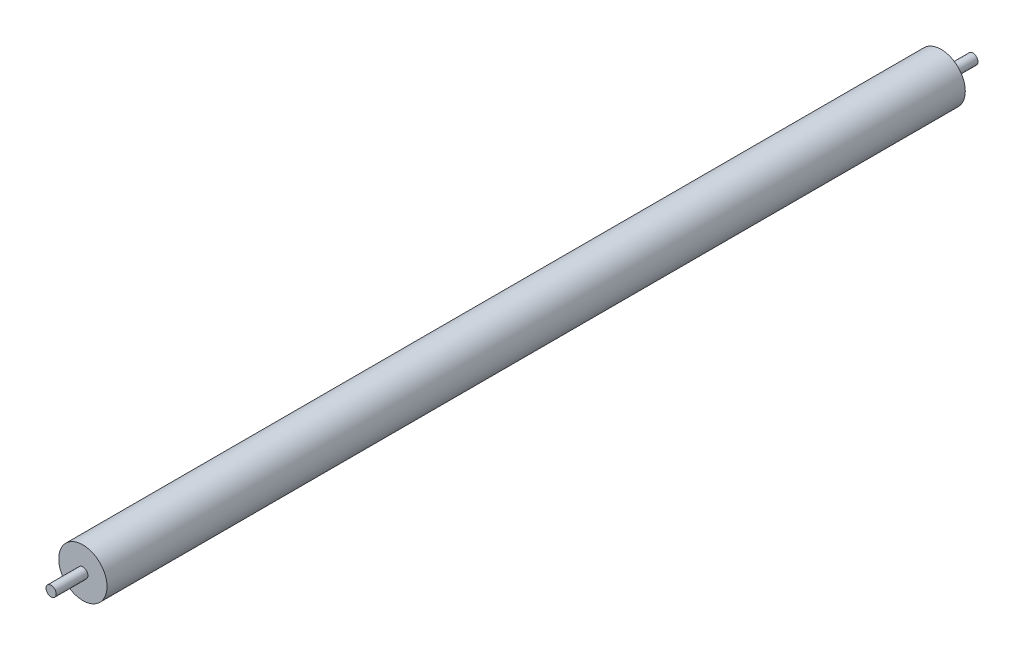
from build123d import *

# Parameters (mm, degrees)
SKETCH_1_R      = 38
EXTRUDE_1_DEPTH = 675
SKETCH_2_R      = 8
EXTRUDE_2_DEPTH = 50


with BuildPart() as part:
    # 草图1 → 凸台-拉伸1 (new, symmetric)
    with BuildSketch(Plane.XY):
        Circle(SKETCH_1_R)
    extrude(amount=EXTRUDE_1_DEPTH, both=True)

    # 草图2 → 凸台-拉伸2 (add, symmetric)
    with BuildSketch(Plane.XY.offset(675)):
        Circle(SKETCH_2_R)
    extrude_2 = extrude(amount=EXTRUDE_2_DEPTH, both=True)

    # 镜向1: 凸台-拉伸2 across plane
    add(extrude_2.mirror(Plane.XY))


solid = part.part
